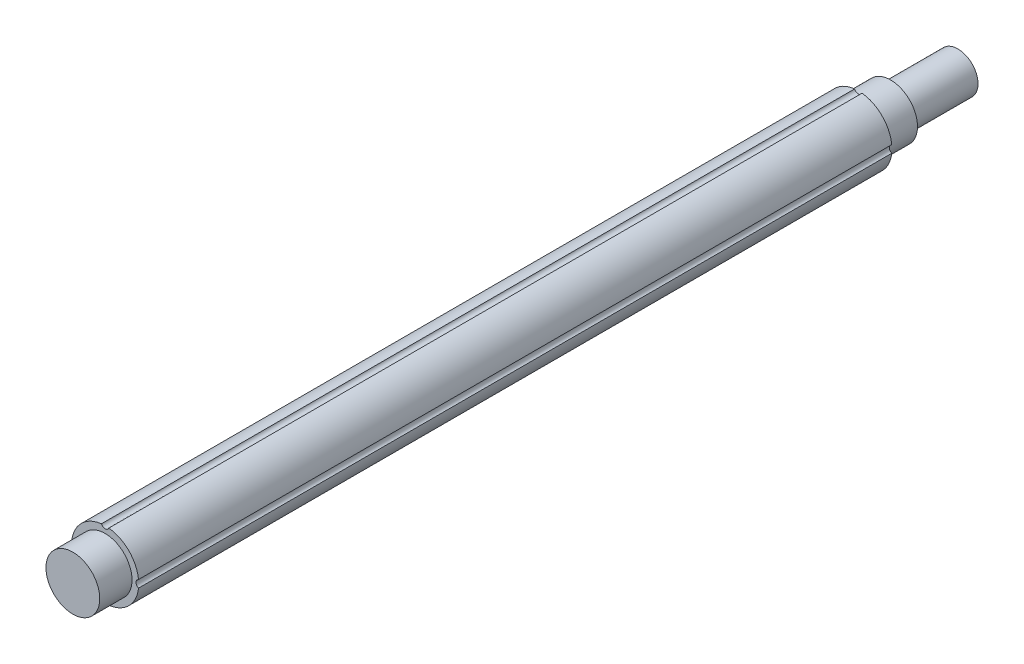
SolidWorks part; units mm, degrees
ref_plane "前视基准面" through (0, 0, 0) normal (0, 0, 1) x (1, 0, 0)
ref_plane "上视基准面" through (0, 0, 0) normal (0, 1, 0) x (1, 0, 0)
ref_plane "右视基准面" through (0, 0, 0) normal (1, 0, 0) x (0, 0, -1)
sketch "草图1" plane through (0, 0, 0) normal (0, 0, 1) x (1, 0, 0)
  circle A0 centre (0, 0) radius 12.5
  dimension "D1" = 25
extrude "凸台-拉伸1" add sketch "草图1" along normal blind 280
sketch "草图2" plane through (0, 0, 280) normal (0, 0, 1) x (1, 0, 0)
  circle A0 centre (0, 0) radius 10
  dimension "D1" = 20
extrude "凸台-拉伸2" add sketch "草图2" along normal blind 12
sketch "草图3" plane through (0, 0, 0) normal (0, 0, -1) x (-1, 0, 0)
  circle A0 centre (0, 0) radius 10
  dimension "D1" = 20
extrude "凸台-拉伸3" add sketch "草图3" along normal blind 12
sketch "草图4" plane through (0, 0, -12) normal (0, 0, -1) x (-1, 0, 0)
  circle A0 centre (0, 0) radius 7.5
  dimension "D1" = 15
extrude "凸台-拉伸4" add sketch "草图4" along normal blind 25
sketch "草图5" plane through (0, 0, 0) normal (0, 0, -1) x (-1, 0, 0)
  circle A0 centre (0, 13) radius 1.5
  dimension "D1" = 3
  dimension "D2" = 13
extrude "切除-拉伸1" cut sketch "草图5" against normal up to surface (280 mm away) up to face at (10, 0, 280)
pattern_circular "阵列(圆周)1" count 4 over 360 about axis through (0, 0, 0) along (0, 0, 1) of "切除-拉伸1"
